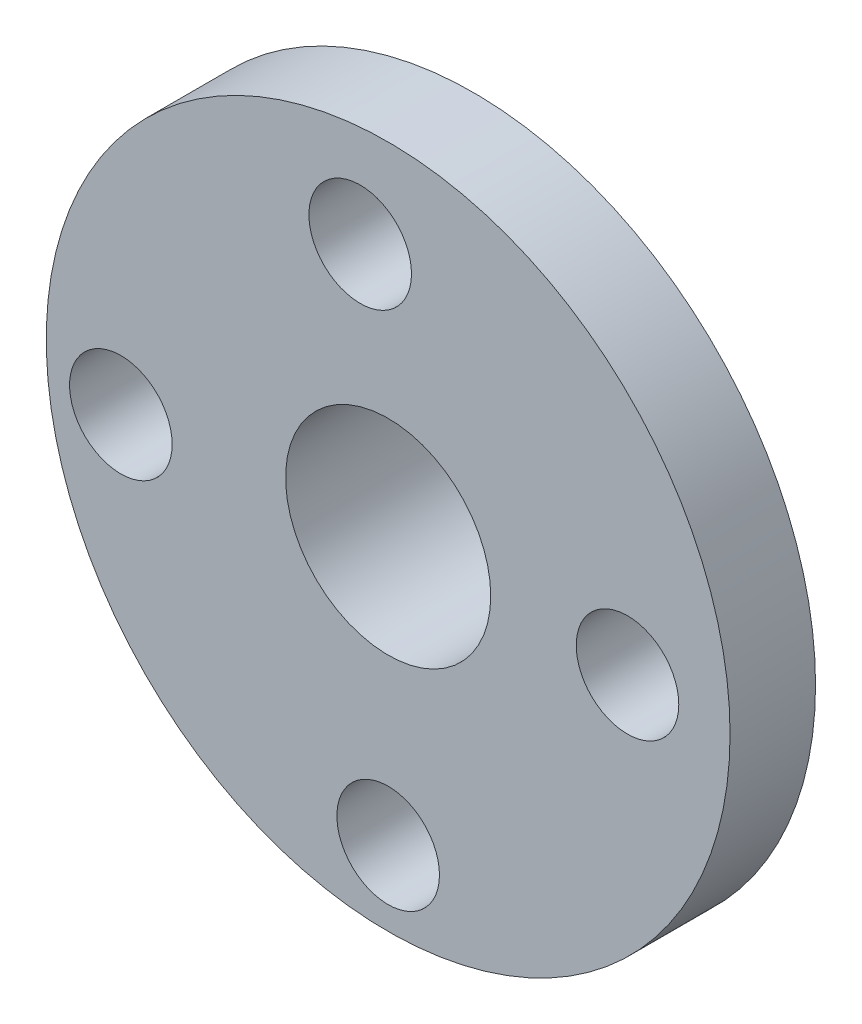
SolidWorks part; units mm, degrees
material "45"
ref_plane "Front Plane" through (0, 0, 0) normal (0, 0, 1) x (1, 0, 0)
ref_plane "Top Plane" through (0, 0, 0) normal (0, 1, 0) x (1, 0, 0)
ref_plane "Right Plane" through (0, 0, 0) normal (1, 0, 0) x (0, 0, -1)
sketch "Sketch3" plane through (0, 0, 0) normal (0, 0, 1) x (1, 0, 0)
  circle A0 centre (0, 0) radius 3
  circle A1 centre (0, 0) radius 4.5
  dimension "D1" = 9
  dimension "D2" = 6
extrude "Boss-Extrude1" add sketch "Sketch3" along normal blind 3
sketch "Sketch4" plane through (0, 0, 3) normal (0, 0, 1) x (1, 0, 0)
  circle A0 centre (0, 0) radius 3
  circle A1 centre (0, 0) radius 10
  dimension "D1" = 6
  dimension "D2" = 20
extrude "Boss-Extrude2" add sketch "Sketch4" along normal blind 2 and the other way blind 0.5
sketch "Sketch5" plane through (0, 0, 5) normal (0, 0, 1) x (1, 0, 0)
  line L0 (-10, 0) -> (49990, 0) construction
  line L1 (-0.8181, 10) -> (-0.8181, 50010) construction
  line L2 (-1.5656, 9.9051) -> (-0.0706, 10.0278) construction
  circle A0 centre (7, 0) radius 1.5
  circle A1 centre (-0.8181, 7) radius 1.5
  circle A2 centre (0, -7.8181) radius 1.5
  circle A3 centre (-7.8181, -0.8181) radius 1.5
  point P6 (-0.8181, 9.9665)
  point P18 (-0.4091, -0.4091)
  dimension "D1" = 3
  dimension "D2" = 14
  dimension "D3" = 4
extrude "Cut-Extrude1" cut sketch "Sketch5" against normal through all
